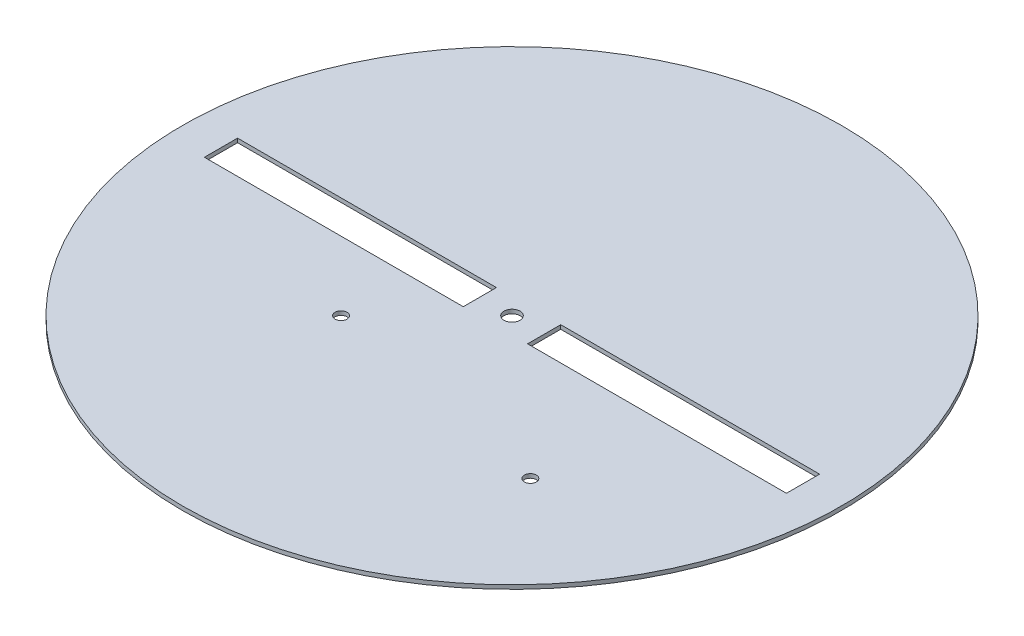
SolidWorks part; units mm, degrees
ref_plane "Front Plane" through (0, 0, 0) normal (0, 0, 1) x (1, 0, 0)
ref_plane "Top Plane" through (0, 0, 0) normal (0, 1, 0) x (1, 0, 0)
ref_plane "Right Plane" through (0, 0, 0) normal (1, 0, 0) x (0, 0, -1)
sketch "Sketch1" plane through (0, 0, 0) normal (0, 1, 0) x (1, 0, 0)
  line L0 (-89.4324, 0) -> (88.3334, 0) construction
  line L1 (0, 91.0809) -> (0, -91.6304) construction
  line L2 (-72.85, 4.15) -> (-8.05, 4.15)
  line L3 (-72.85, 4.15) -> (-72.85, -4.15)
  line L4 (-72.85, -4.15) -> (-8.05, -4.15)
  line L5 (-8.05, 4.15) -> (-8.05, -4.15)
  line L6 (8.05, 4.15) -> (8.05, -4.15)
  line L7 (72.85, -4.15) -> (8.05, -4.15)
  line L8 (72.85, 4.15) -> (72.85, -4.15)
  line L9 (72.85, 4.15) -> (8.05, 4.15)
  circle A0 centre (0, 0) radius 82.5
  circle A1 centre (-21.4, -21.4) radius 1.5
  circle A2 centre (37.6, -33) radius 1.5
  circle A3 centre (0, 0) radius 2
  dimension "D1" = 165
  dimension "D7" = 3
  dimension "D9" = 33
  dimension "D10" = 4
  dimension "D2" = 8.3
  dimension "D3" = 64.8
  dimension "D4" = 16.1
  dimension "D5" = 21.4
  dimension "D6" = 21.4
  dimension "D8" = 37.6
extrude "Boss-Extrude1" add sketch "Sketch1" along normal blind 1
